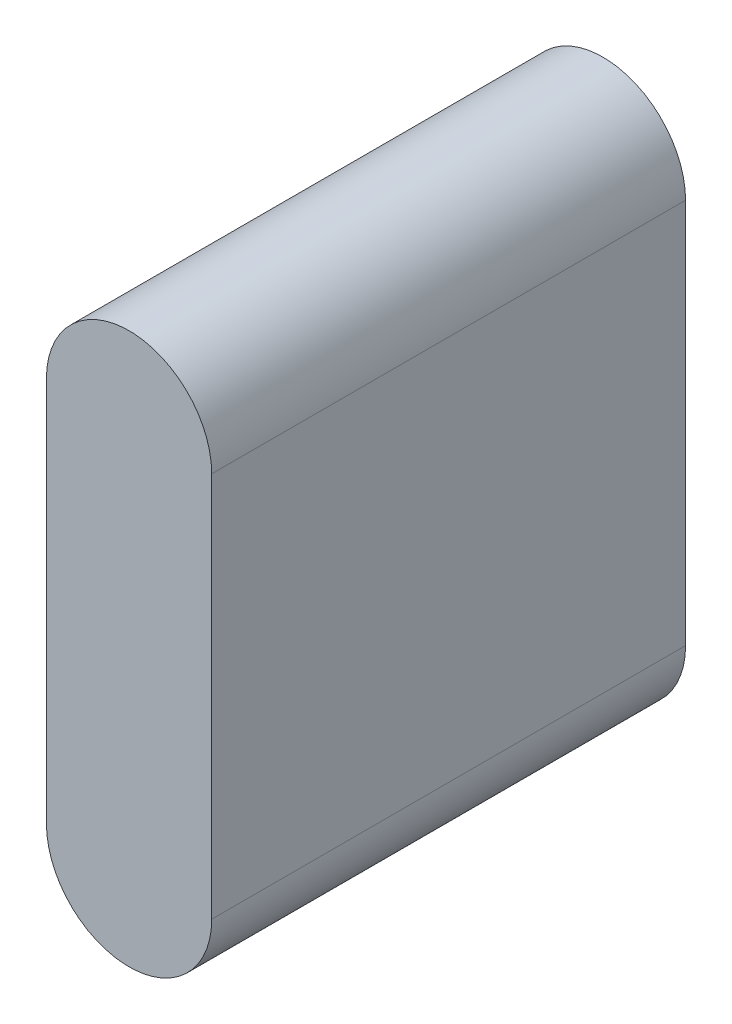
from build123d import *

# Parameters (mm, degrees)
EXTRUDE_1_DEPTH = 2.15


with BuildPart() as part:
    # 草图1 → 凸台-拉伸1 (new, symmetric)
    with BuildSketch(Plane.XY):
        with BuildLine():
            Line((-0.75, -1.75), (-0.75, 1.75))
            ThreePointArc((-0.75, 1.75), (0, 2.5), (0.75, 1.75))
            Line((0.75, 1.75), (0.75, -1.75))
            ThreePointArc((0.75, -1.75), (0, -2.5), (-0.75, -1.75))
        make_face()
    extrude(amount=EXTRUDE_1_DEPTH, both=True)


solid = part.part
